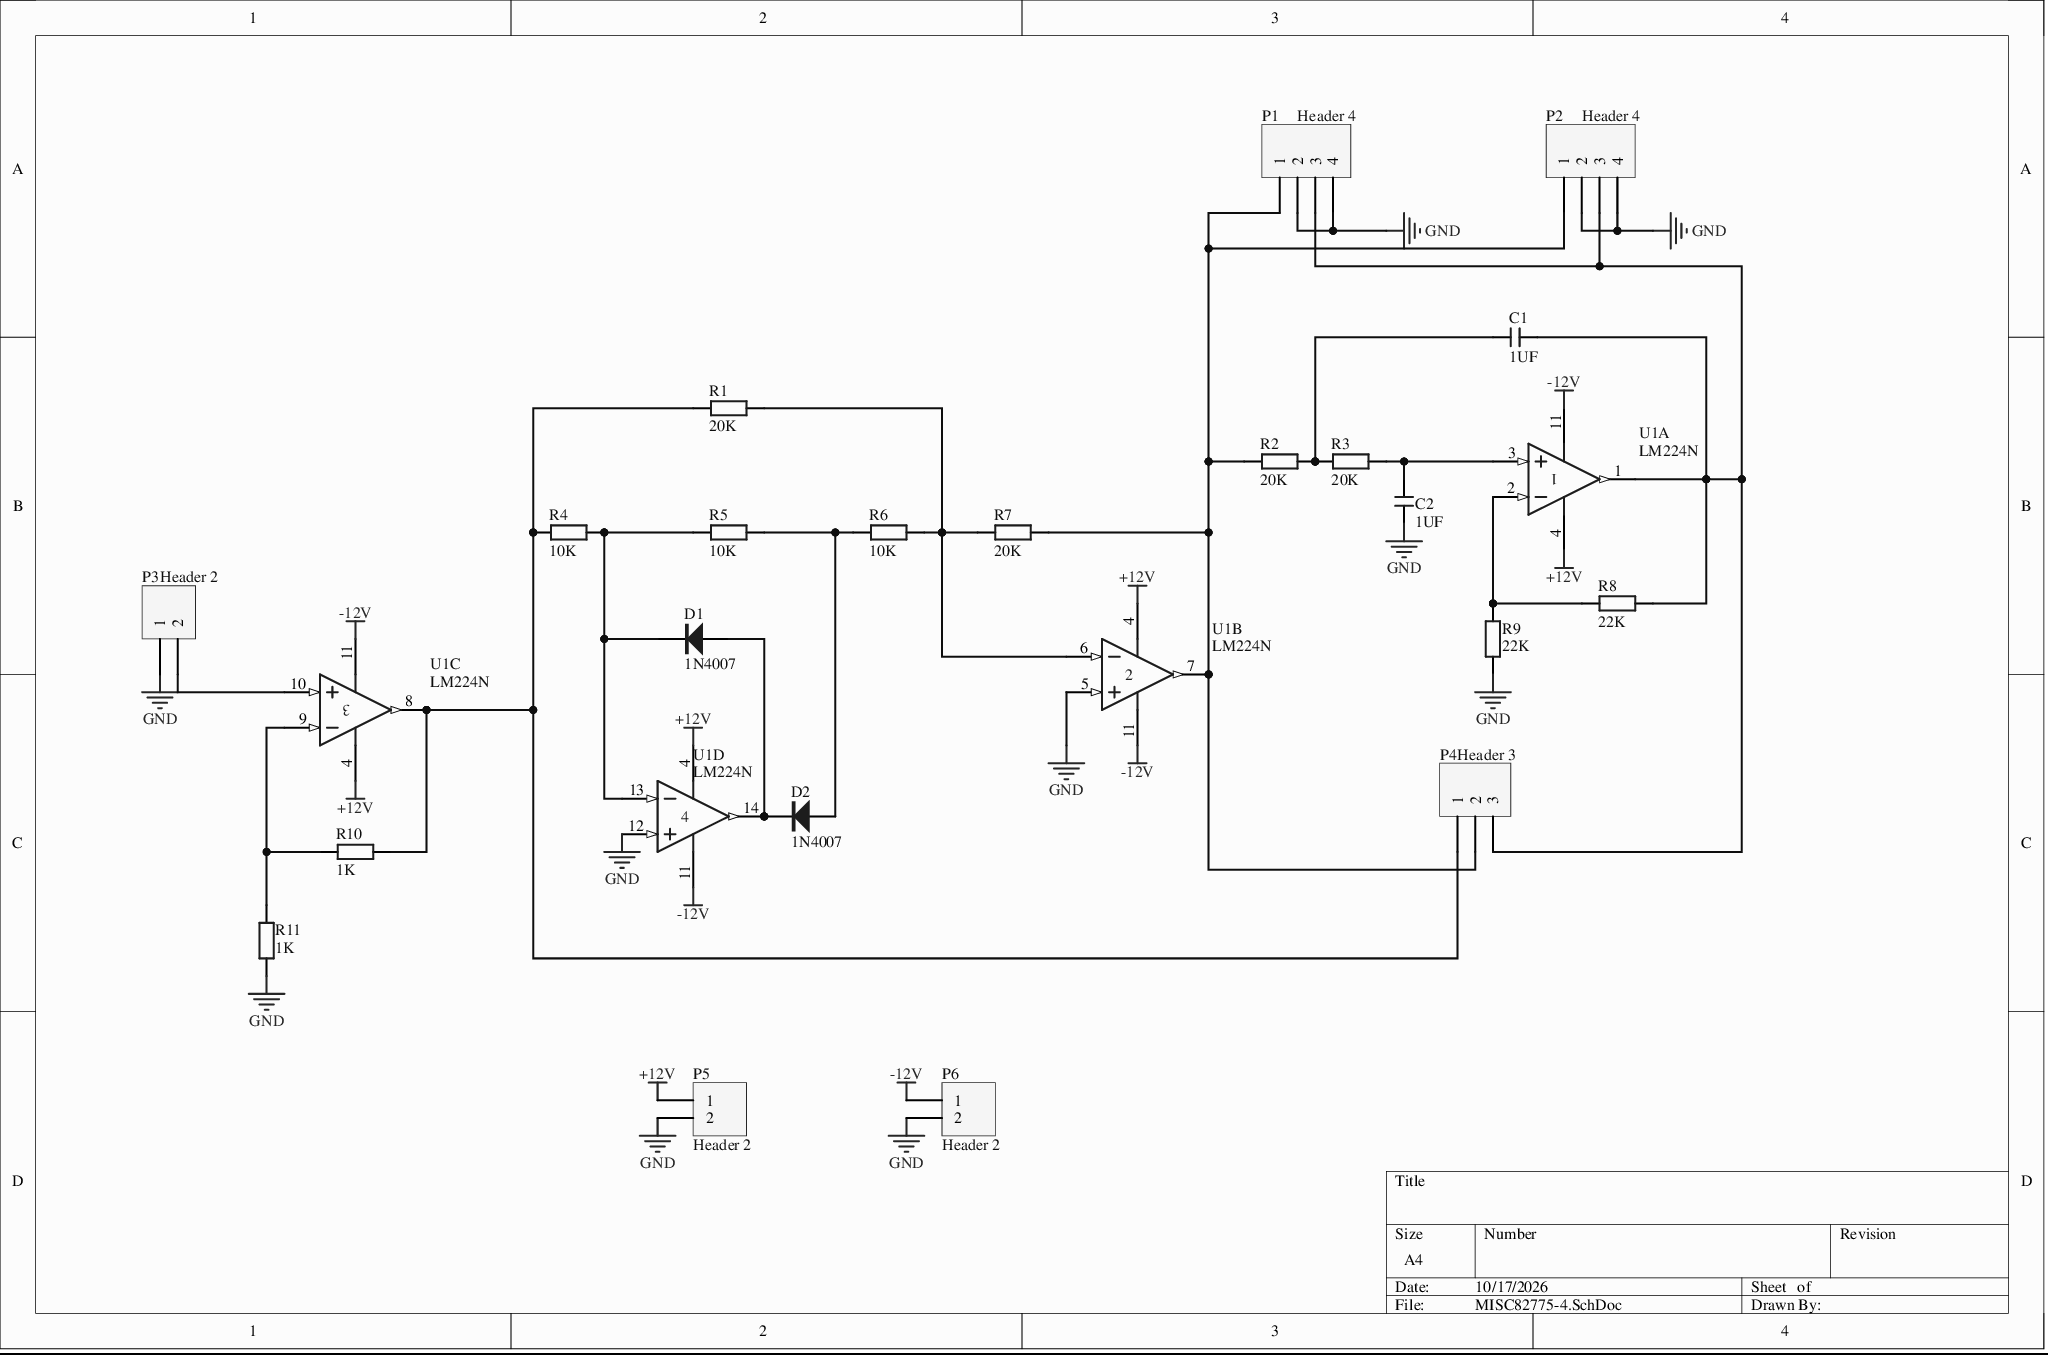
[diagram p0: MISC82775-4.SchDoc]
# Altium project MISC82775-7.PrjPcb
1 sheet, 22 parts. Net scope: global (net labels, ports and power ports of the same name join across sheets).
Board file: MISC82775.PcbDoc

## Sheet MISC82775-4.SchDoc
size A4

### Parts
C1  1UF  [CC 1.8*3.6]
C2  1UF  [CC 1.8*3.6]
D1  1N4007  [DO-41]
D2  1N4007  [DO-41]
P1  Header 4  [HDR1X4]
P2  Header 4  [HDR1X4]
P3  Header 2  [HDR1X2]
P4  Header 3  [HDR1X3]
P5  Header 2  [HDR1X2]
P6  Header 2  [HDR1X2]
R1  20K  [RS 1/4W]
R2  20K  [RS 1/4W]
R3  20K  [RS 1/4W]
R4  10K  [RS 1/4W]
R5  10K  [RS 1/4W]
R6  10K  [RS 1/4W]
R7  20K  [RS 1/4W]
R8  22K  [RS 1/4W]
R9  22K  [RS 1/4W]
R10  1K  [RS 1/4W]
R11  1K  [RS 1/4W]
U1  LM224N  [646-06]  (parts A,B,C,D of 4)

### Nets
+12V: P5.1 U1.4(V+)
-12V: P6.1 U1.11(V-)
GND: C2.2 P1.2 P1.4 P2.2 P2.4 P3.1 P5.2 P6.2 R9.1 R11.1 U1.5(IN+) U1.12(IN+)
NetC1_1: C1.1 R2.2 R3.1
NetC1_2: C1.2 P1.3 P2.3 P4.3 R8.2 U1.1(OUT)
NetC2_1: C2.1 R3.2 U1.3(IN+)
NetD1_1: D1.1(A) D2.2(K) U1.14(OUT)
NetD1_2: D1.2(K) R4.2 R5.1 U1.13(IN-)
NetD2_1: D2.1(A) R5.2 R6.1
NetP1_1: P1.1 P2.1 P4.2 R2.1 R7.2 U1.7(OUT)
NetP3_2: P3.2 U1.10(IN+)
NetP4_1: P4.1 R1.1 R4.1 R10.2 U1.8(OUT)
NetR1_2: R1.2 R6.2 R7.1 U1.6(IN-)
NetR8_1: R8.1 R9.2 U1.2(IN-)
NetR10_1: R10.1 R11.2 U1.9(IN-)

### Library data of the parts
C1 C2 = CC: Ceramic capacitor; BOM名称: Through-hole ceramic capacitor
D1 D2 = 1N4007: Rectifier diode; BOM名称: Rectifier diode
P1 P2 = Header 4: Header, 4-Pin; LatestRevisionDate: 17-Jul-2002; LatestRevisionNote: Re-released for DXP Platform.; Publisher: Altium Limited
P3 P5 P6 = Header 2: Header, 2-Pin; LatestRevisionDate: 17-Jul-2002; LatestRevisionNote: Re-released for DXP Platform.; Publisher: Altium Limited
P4 = Header 3: Header, 3-Pin; LatestRevisionDate: 17-Jul-2002; LatestRevisionNote: Re-released for DXP Platform.; Publisher: Altium Limited
R1-R11 = R-S: Color-band resistor; BOM名称: Color-band resistor
U1 = LM224N: Quad Low-Power Operational Amplifier; Package Information: Latest Revision: 1997; Published: 17-Jul-2002; Datasheet: Linear and Interface Integrated Circuits, DL128 Rev2 (1988); Package Reference: 646-06; Publisher: Altium Limited